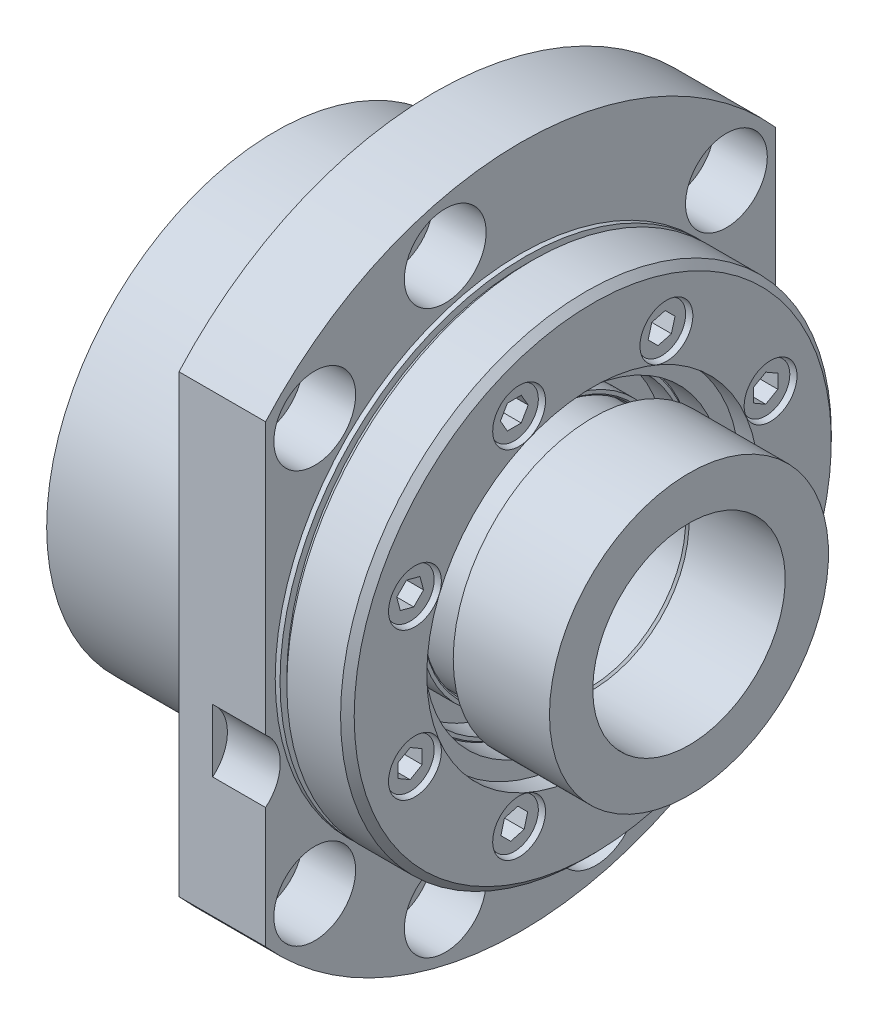
from build123d import *

# Parameters (mm, degrees)
SKETCH_2_R                  = 81
CUT_EXTRUDE_1_DEPTH         = 66
SKETCH_3_R                  = 8.5
CUT_EXTRUDE_2_DEPTH         = 11
PATTERN_CIRCULAR_1_COUNT    = 10
PATTERN_CIRCULAR_1_ANGLE    = 270
SKETCH_5_R                  = 5.5
CUT_EXTRUDE_3_DEPTH         = 11
SKETCH_7_R                  = 5.5
CUT_EXTRUDE_4_DEPTH         = 11
SKETCH_8_R                  = 5.5
CUT_EXTRUDE_5_DEPTH         = 11
SKETCH_9_R                  = 5.5
CUT_EXTRUDE_6_DEPTH         = 11
SKETCH_10_R                 = 5.5
CUT_EXTRUDE_7_DEPTH         = 11
SKETCH_11_R                 = 5.5
CUT_EXTRUDE_8_DEPTH         = 11
SKETCH_12_R                 = 5.5
CUT_EXTRUDE_9_DEPTH         = 11
SKETCH_13_R                 = 5.5
CUT_EXTRUDE_10_DEPTH        = 11
PATTERN_LINEAR_1_COUNT      = 2
PATTERN_LINEAR_1_PITCH      = 56.568542495
PATTERN_LINEAR_1_COUNT_DIR2 = 2
PATTERN_LINEAR_1_PITCH_DIR2 = 56.568542495
SKETCH_18_R                 = 5.49
CUT_EXTRUDE_11_DEPTH        = 7
PATTERN_CIRCULAR_3_COUNT    = 8
SKETCH_20_R                 = 5
EXTRUDE_1_DEPTH             = 6
PATTERN_CIRCULAR_4_COUNT    = 8
CUT_EXTRUDE_12_DEPTH        = 4
PATTERN_CIRCULAR_5_COUNT    = 8
SKETCH_26_W                 = 20
SKETCH_26_H                 = 9
SKETCH_29_R                 = 8.5
EXTRUDE_2_DEPTH             = 11


with BuildPart() as part:
    # 草图1 → 旋转1 (revolve)
    with BuildSketch(Plane.XY, mode=Mode.PRIVATE) as revolve_1_sk:
        Polygon((0, 47.5), (0, 34.5), (4, 34.5), (4, 31), (11, 31), (11, 30.5), (18, 30.5), (18, 36), (50.585786438, 36), (52, 37.414213562), (52, 51), (51, 51), (51, 71), (33, 71), (33, 47.5), align=None)
    revolve(revolve_1_sk.sketch.rotate(Axis((50, 0, 0), (-1, 0, 0)), 270), axis=Axis((50, 0, 0), (-1, 0, 0)))

    # 草图2 → 切除-拉伸1 (cut)
    with BuildSketch(Plane(origin=(0, 0, 0), x_dir=(0, 0, -1), z_dir=(1, 0, 0))):
        Circle(SKETCH_2_R)
        with BuildLine():
            Line((-53, 47.244047244), (-53, -47.244047244))
            ThreePointArc((-53, -47.244047244), (0, -71), (53, -47.244047244))
            Line((53, -47.244047244), (53, 47.244047244))
            ThreePointArc((53, 47.244047244), (0, 71), (-53, 47.244047244))
        make_face(mode=Mode.SUBTRACT)
    extrude(amount=CUT_EXTRUDE_1_DEPTH, mode=Mode.SUBTRACT)

    # 草图3 → 切除-拉伸2 (cut)
    with BuildSketch(Plane(origin=(51, 0, 0), x_dir=(0, 0, -1), z_dir=(1, 0, 0))):
        with Locations((42.779960262, 42.779960262)):
            Circle(SKETCH_3_R)
    cut_extrude_2 = extrude(amount=-CUT_EXTRUDE_2_DEPTH, mode=Mode.SUBTRACT)

    # 阵列(圆周)1: 切除-拉伸2 ×10 about axis, 2 skipped
    pattern_circular_1_axis = Axis((51, 0, 0), (1, 0, 0))
    add([cut_extrude_2.rotate(pattern_circular_1_axis, i * PATTERN_CIRCULAR_1_ANGLE / (PATTERN_CIRCULAR_1_COUNT - 1)) for i in range(1, PATTERN_CIRCULAR_1_COUNT) if i not in (1, 4)], mode=Mode.SUBTRACT)

    # 草图5 → 切除-拉伸3 (cut)
    with BuildSketch(Plane(origin=(40, 0, 0), x_dir=(0, 0, -1), z_dir=(1, 0, 0))):
        with Locations((42.779960262, 42.779960262)):
            Circle(SKETCH_5_R)
    extrude(amount=-CUT_EXTRUDE_3_DEPTH, mode=Mode.SUBTRACT)

    # 草图7 → 切除-拉伸4 (cut)
    with BuildSketch(Plane(origin=(40, 0, 0), x_dir=(0, 0, -1), z_dir=(1, 0, 0))):
        with Locations((15.658552229, 58.43851249)):
            Circle(SKETCH_7_R)
    extrude(amount=-CUT_EXTRUDE_4_DEPTH, mode=Mode.SUBTRACT)

    # 草图8 → 切除-拉伸5 (cut)
    with BuildSketch(Plane(origin=(40, 0, 0), x_dir=(0, 0, -1), z_dir=(1, 0, 0))):
        with Locations((-15.658552229, 58.43851249)):
            Circle(SKETCH_8_R)
    extrude(amount=-CUT_EXTRUDE_5_DEPTH, mode=Mode.SUBTRACT)

    # 草图9 → 切除-拉伸6 (cut)
    with BuildSketch(Plane(origin=(40, 0, 0), x_dir=(0, 0, -1), z_dir=(1, 0, 0))):
        with Locations((-42.779960262, 42.779960262)):
            Circle(SKETCH_9_R)
    extrude(amount=-CUT_EXTRUDE_6_DEPTH, mode=Mode.SUBTRACT)

    # 草图10 → 切除-拉伸7 (cut)
    with BuildSketch(Plane(origin=(40, 0, 0), x_dir=(0, 0, -1), z_dir=(1, 0, 0))):
        with Locations((-42.779960262, -42.779960262)):
            Circle(SKETCH_10_R)
    extrude(amount=-CUT_EXTRUDE_7_DEPTH, mode=Mode.SUBTRACT)

    # 草图11 → 切除-拉伸8 (cut)
    with BuildSketch(Plane(origin=(40, 0, 0), x_dir=(0, 0, -1), z_dir=(1, 0, 0))):
        with Locations((-15.658552229, -58.43851249)):
            Circle(SKETCH_11_R)
    extrude(amount=-CUT_EXTRUDE_8_DEPTH, mode=Mode.SUBTRACT)

    # 草图12 → 切除-拉伸9 (cut)
    with BuildSketch(Plane(origin=(40, 0, 0), x_dir=(0, 0, -1), z_dir=(1, 0, 0))):
        with Locations((15.658552229, -58.43851249)):
            Circle(SKETCH_12_R)
    extrude(amount=-CUT_EXTRUDE_9_DEPTH, mode=Mode.SUBTRACT)

    # 草图13 → 切除-拉伸10 (cut)
    with BuildSketch(Plane(origin=(40, 0, 0), x_dir=(0, 0, -1), z_dir=(1, 0, 0))):
        with Locations((42.779960262, -42.779960262)):
            Circle(SKETCH_13_R)
    extrude(amount=-CUT_EXTRUDE_10_DEPTH, mode=Mode.SUBTRACT)

    # 草图14 → 切除-旋转1 (revolve, cut)
    with BuildSketch(Plane.XY, mode=Mode.PRIVATE) as cut_revolve_1_sk:
        Polygon((0, 40), (0, 43), (0.5415, 42.4585), (11.4585, 42.4585), (12, 43), (12, 40), align=None)
    cut_revolve_1 = revolve(cut_revolve_1_sk.sketch.rotate(Axis((12, 40, 0), (-1, 0, 0)), 270), axis=Axis((12, 40, 0), (-1, 0, 0)), mode=Mode.SUBTRACT)

    # 阵列(线性)1: Cut-Revolve 1 2 × 2
    with Locations(*[Vector(0, -0.7071067811865475, 0.7071067811865477) * (i * PATTERN_LINEAR_1_PITCH) + Vector(0, -0.7071067811865477, -0.7071067811865474) * (j * PATTERN_LINEAR_1_PITCH_DIR2) for i in range(PATTERN_LINEAR_1_COUNT) for j in range(PATTERN_LINEAR_1_COUNT_DIR2) if (i, j) != (0, 0)]):
        add(cut_revolve_1, mode=Mode.SUBTRACT)

    # 草图16 → 旋转2 (revolve)
    with BuildSketch(Plane.XY, mode=Mode.PRIVATE) as revolve_2_sk:
        Polygon((18, 34.585786438), (18, 21.414213562), (19.414213562, 20), (31.585786438, 20), (33, 21.414213562), (34.414213562, 20), (46.585786438, 20), (48, 21.414213562), (48, 34.585786438), (46.585786438, 36), (34.414213562, 36), (33, 34.585786438), (31.585786438, 36), (19.414213562, 36), align=None)
    revolve(revolve_2_sk.sketch.rotate(Axis((50, 0, 0), (-1, 0, 0)), 270), axis=Axis((50, 0, 0), (-1, 0, 0)))

    # 草图17 → 旋转3 (revolve)
    with BuildSketch(Plane.XY, mode=Mode.PRIVATE) as revolve_3_sk:
        Polygon((48, 34.585786438), (48, 32.414213562), (49.414213562, 31), (62, 31), (62, 34.5), (66, 34.5), (66, 49.585786438), (64.585786438, 51), (53.414213562, 51), (52, 49.585786438), (52, 36), (49.414213562, 36), align=None)
    revolve(revolve_3_sk.sketch.rotate(Axis((50, 0, 0), (-1, 0, 0)), 270), axis=Axis((50, 0, 0), (-1, 0, 0)))

    # 草图18 → 切除-拉伸11 (cut)
    with BuildSketch(Plane(origin=(66, 0, 0), x_dir=(0, 0, -1), z_dir=(1, 0, 0))):
        with Locations((36.9551813, 15.307337295)):
            Circle(SKETCH_18_R)
    cut_extrude_11 = extrude(amount=-CUT_EXTRUDE_11_DEPTH, mode=Mode.SUBTRACT)

    # 阵列(圆周)3: 切除-拉伸11 ×8 about axis
    pattern_circular_3_axis = Axis((0, 0, 0), (1, 0, 0))
    for i in range(1, PATTERN_CIRCULAR_3_COUNT):
        add(cut_extrude_11.rotate(pattern_circular_3_axis, i * 360 / PATTERN_CIRCULAR_3_COUNT), mode=Mode.SUBTRACT)

    # 草图20 → 凸台-拉伸1 (add)
    with BuildSketch(Plane(origin=(65, 0, 0), x_dir=(0, 0, -1), z_dir=(1, 0, 0))):
        with Locations((36.9551813, 15.307337295)):
            Circle(SKETCH_20_R)
    extrude_1 = extrude(amount=-EXTRUDE_1_DEPTH)

    # 阵列(圆周)4: 凸台-拉伸1 ×8 about axis
    pattern_circular_4_axis = Axis((0, 0, 0), (1, 0, 0))
    for i in range(1, PATTERN_CIRCULAR_4_COUNT):
        add(extrude_1.rotate(pattern_circular_4_axis, i * 360 / PATTERN_CIRCULAR_4_COUNT))

    # 草图22 → 切除-拉伸12 (cut)
    with BuildSketch(Plane(origin=(65, 0, 0), x_dir=(0, 0, -1), z_dir=(1, 0, 0))):
        Polygon((34.4551813, 13.863961622), (36.9551813, 12.420585949), (39.4551813, 13.863961622), (39.4551813, 16.750712968), (36.9551813, 18.194088641), (34.4551813, 16.750712968), align=None)
    cut_extrude_12 = extrude(amount=-CUT_EXTRUDE_12_DEPTH, mode=Mode.SUBTRACT)

    # 阵列(圆周)5: 切除-拉伸12 ×8 about axis
    pattern_circular_5_axis = Axis((0, 0, 0), (1, 0, 0))
    for i in range(1, PATTERN_CIRCULAR_5_COUNT):
        add(cut_extrude_12.rotate(pattern_circular_5_axis, i * 360 / PATTERN_CIRCULAR_5_COUNT), mode=Mode.SUBTRACT)

    # 草图24 → 旋转4 (revolve)
    with BuildSketch(Plane.XY, mode=Mode.PRIVATE) as revolve_4_sk:
        Polygon((0, 23.992893219), (0, 20.707106781), (0.707106781, 20), (17.292893219, 20), (18, 20.707106781), (18, 23.992893219), (17.292893219, 24.7), (0.707106781, 24.7), align=None)
    revolve(revolve_4_sk.sketch.rotate(Axis((50, 0, 0), (-1, 0, 0)), 270), axis=Axis((50, 0, 0), (-1, 0, 0)))

    # 草图25 → 旋转5 (revolve)
    with BuildSketch(Plane.XY, mode=Mode.PRIVATE) as revolve_5_sk:
        Polygon((4, 30.717157288), (4, 30), (9, 30), (9, 26), (4, 26), (4, 25.282842712), (4.282842712, 25), (9.292893219, 25), (10, 25.707106781), (10, 30.292893219), (9.292893219, 31), (4.282842712, 31), align=None)
    revolve(revolve_5_sk.sketch.rotate(Axis((50, 0, 0), (-1, 0, 0)), 270), axis=Axis((50, 0, 0), (-1, 0, 0)))

    # 草图27 → 旋转6 (revolve)
    with BuildSketch(Plane.XY, mode=Mode.PRIVATE) as revolve_6_sk:
        Polygon((48, 23.992893219), (48, 20.707106781), (48.707106781, 20), (65.292893219, 20), (66, 20.707106781), (66, 23.992893219), (65.292893219, 24.7), (48.707106781, 24.7), align=None)
    revolve(revolve_6_sk.sketch.rotate(Axis((50, 0, 0), (-1, 0, 0)), 270), axis=Axis((50, 0, 0), (-1, 0, 0)))

    # 草图26 → 旋转7 (revolve)
    with BuildSketch(Plane.XY, mode=Mode.PRIVATE) as revolve_7_sk:
        with Locations((76, 24.5)):
            Rectangle(SKETCH_26_W, SKETCH_26_H)
    revolve(revolve_7_sk.sketch.rotate(Axis((50, 0, 0), (-1, 0, 0)), 90), axis=Axis((50, 0, 0), (-1, 0, 0)))

    # 草图28 → 旋转8 (revolve)
    with BuildSketch(Plane.XY, mode=Mode.PRIVATE) as revolve_8_sk:
        Polygon((50, 30.292893219), (50, 25.707106781), (50.707106781, 25), (55.717157288, 25), (56, 25.282842712), (56, 26), (51, 26), (51, 30), (56, 30), (56, 30.717157288), (55.717157288, 31), (50.707106781, 31), align=None)
    revolve(revolve_8_sk.sketch.rotate(Axis((50, 0, 0), (-1, 0, 0)), 270), axis=Axis((50, 0, 0), (-1, 0, 0)))

    # 草图29 → 凸台-拉伸2 (add)
    with BuildSketch(Plane(origin=(51, 0, 0), x_dir=(0, 0, -1), z_dir=(1, 0, 0))):
        with Locations((15.658552229, 58.43851249)):
            Circle(SKETCH_29_R)
    extrude(amount=-EXTRUDE_2_DEPTH)


solid = part.part
